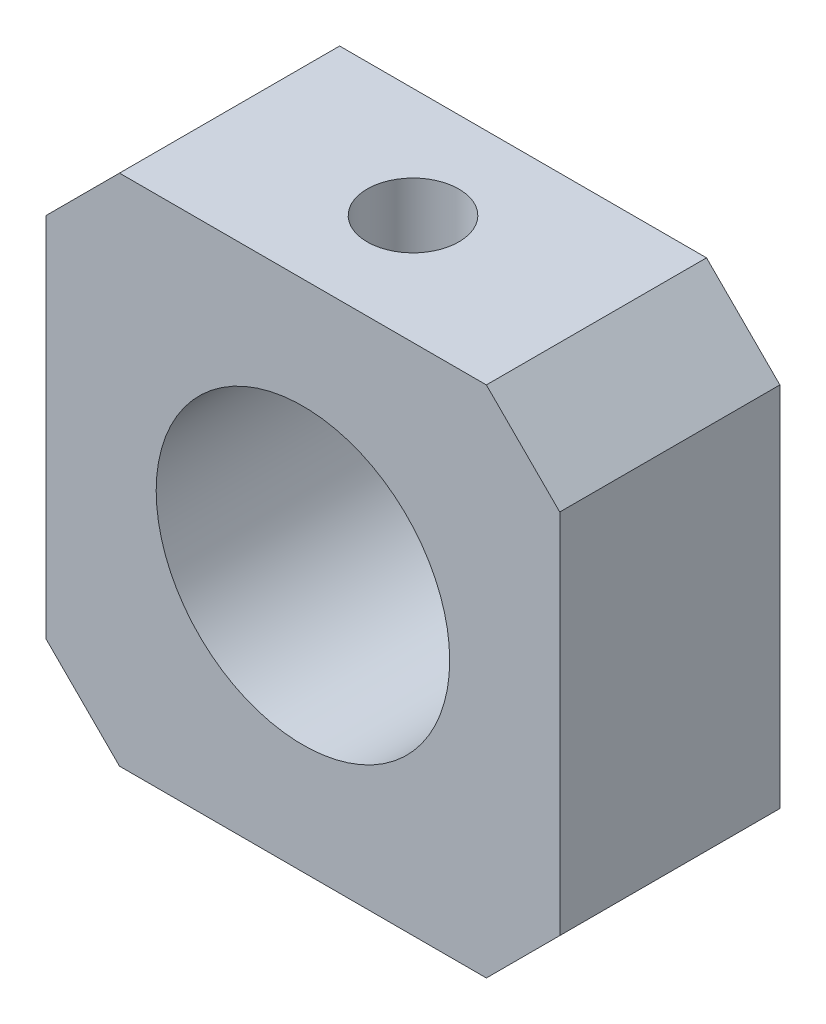
from build123d import *

# Parameters (mm, degrees)
SKETCH_1_W              = 14
SKETCH_1_H              = 14
SKETCH_1_R              = 4
EXTRUDE_1_DEPTH         = 3
HOLE_WIZARD_M3_1_REACH  = 17.937
HOLE_WIZARD_M3_1_BORE_R = 1.25
CHAMFER_2_SIZE          = 2


with BuildPart() as part:
    # 草图1 → 凸台-拉伸1 (new, symmetric)
    with BuildSketch(Plane.XY):
        Rectangle(SKETCH_1_W, SKETCH_1_H)
        Circle(SKETCH_1_R, mode=Mode.SUBTRACT)
    extrude(amount=EXTRUDE_1_DEPTH, both=True)

    # M3 螺纹孔1 bore (on position points) → M3 螺纹孔1 (cut, up to next)
    with BuildSketch(Plane.ZX.offset(7), mode=Mode.PRIVATE) as hole_wizard_m3_1_sk1:
        Circle(HOLE_WIZARD_M3_1_BORE_R)
    hole_wizard_m3_1_tool1 = extrude(hole_wizard_m3_1_sk1.sketch, amount=-HOLE_WIZARD_M3_1_REACH, mode=Mode.PRIVATE) & part.part
    add(hole_wizard_m3_1_tool1.solids().sort_by_distance((0, 7, 0))[0], mode=Mode.SUBTRACT)

    # 倒角2
    chamfer_2_edges = [part.edges().sort_by_distance(p)[0] for p in [
        (7, -7, 0),
        (-7, -7, 0),
        (-7, 7, 0),
        (7, 7, 0),
    ]]
    chamfer(chamfer_2_edges, length=CHAMFER_2_SIZE)


solid = part.part
